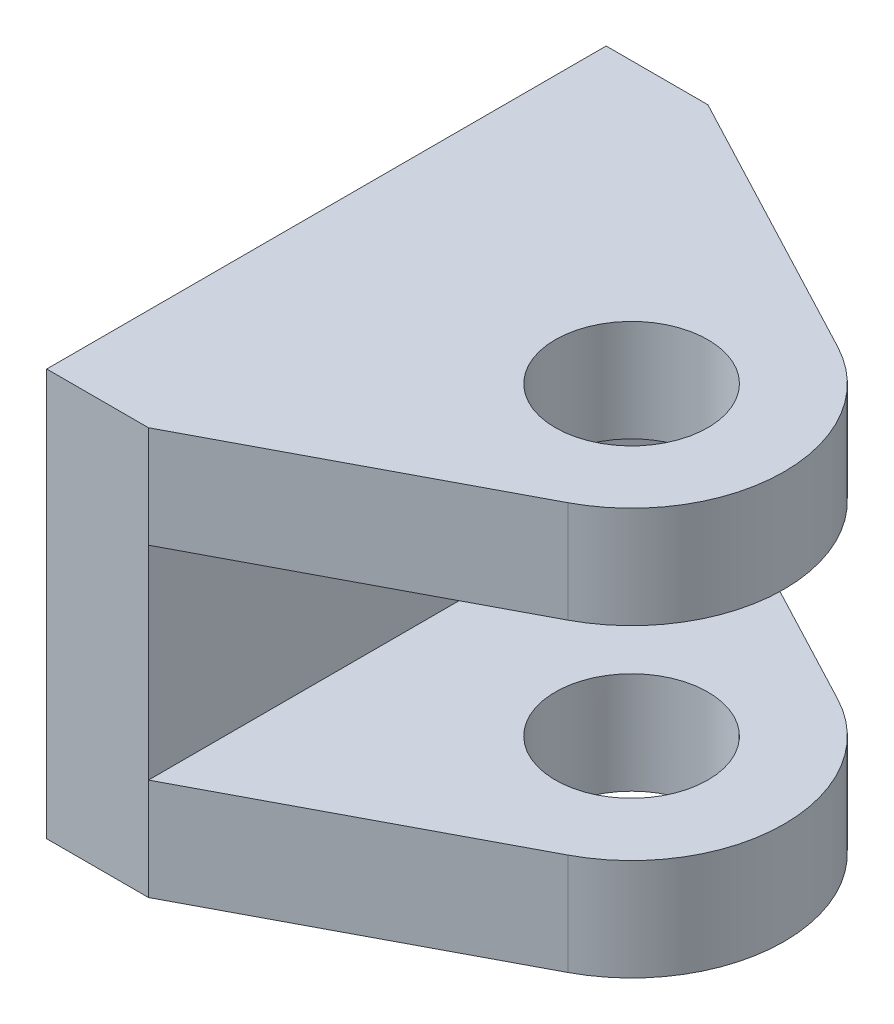
from build123d import *

# Parameters (mm, degrees)
SKETCH_1_R             = 7.5
EXTRUDE_1_DEPTH        = 40
SKETCH_2_W             = 54.950775634
SKETCH_2_H             = 20
CUT_EXTRUDE_1_DEPTH    = 82.547532152
HOLE_WIZARD_M6_1_D     = 5
HOLE_WIZARD_M6_1_DEPTH = 15
HOLE_WIZARD_M6_1_TIP   = 1.502151548


with BuildPart() as part:
    # 草图1 → 凸台-拉伸1 (new body)
    with BuildSketch(Plane(origin=(0, 0, 0), x_dir=(1, 0, 0), z_dir=(0, 1, 0))):
        with BuildLine():
            Line((0, -27.5), (0, 27.5))
            Line((0, 27.5), (10, 27.5))
            Line((10, 27.5), (36.99503609, 13.269117156))
            ThreePointArc((36.99503609, 13.269117156), (45, 0), (36.99503609, -13.269117156))
            Line((36.99503609, -13.269117156), (10, -27.5))
            Line((10, -27.5), (0, -27.5))
        make_face()
        with Locations(Location((30, 0, 0), (0, 0, 270))):
            Circle(SKETCH_1_R, mode=Mode.SUBTRACT)
    extrude(amount=EXTRUDE_1_DEPTH)

    # 草图2 → 切除-拉伸1 (cut, through all)
    with BuildSketch(Plane(origin=(0, 0, -27.5), x_dir=(-1, 0, 0), z_dir=(0, 0, -1))):
        with Locations((-37.475387817, 20)):
            Rectangle(SKETCH_2_W, SKETCH_2_H)
    extrude(amount=-CUT_EXTRUDE_1_DEPTH, mode=Mode.SUBTRACT)

    # M6 螺纹孔1
    with Locations(Plane.ZY):
        with Locations((-19.5, 5), (-19.5, 35), (19.5, 5), (19.5, 35)):
            Hole(HOLE_WIZARD_M6_1_D / 2, depth=HOLE_WIZARD_M6_1_DEPTH)
            with Locations((0, 0, -(HOLE_WIZARD_M6_1_DEPTH + HOLE_WIZARD_M6_1_TIP / 2))):  # 118° drill point
                Cone(0, HOLE_WIZARD_M6_1_D / 2, HOLE_WIZARD_M6_1_TIP, mode=Mode.SUBTRACT)


solid = part.part
